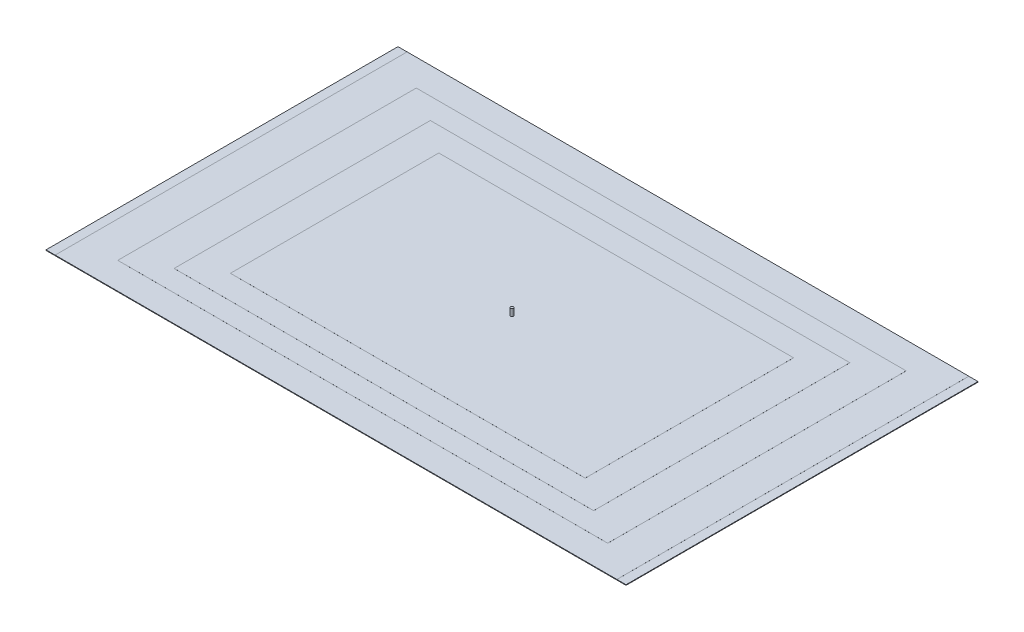
from build123d import *

# Parameters (mm, degrees)
SKETCH_1_W      = 2060
SKETCH_1_H      = 1250
EXTRUDE_1_DEPTH = 1
SKETCH_2_W      = 1995
SKETCH_2_H      = 1250
EXTRUDE_2_DEPTH = 0.1
SKETCH_3_W      = 1740
SKETCH_3_H      = 1060
EXTRUDE_5_DEPTH = 0.1
SKETCH_4_W      = 1490
SKETCH_4_H      = 910
EXTRUDE_6_DEPTH = 0.1
SKETCH_5_W      = 1260
SKETCH_5_H      = 740
EXTRUDE_7_DEPTH = 0.1
SKETCH_6_R      = 5
EXTRUDE_8_DEPTH = 25


with BuildPart() as part:
    # 草图1 → 凸台-拉伸1 (new, symmetric)
    with BuildSketch(Plane(origin=(0, 0, 0), x_dir=(1, 0, 0), z_dir=(0, 1, 0))):
        Rectangle(SKETCH_1_W, SKETCH_1_H)
    extrude(amount=EXTRUDE_1_DEPTH, both=True)


with BuildPart() as body_2:
    # 草图2 → 凸台-拉伸2 (new body)
    with BuildSketch(Plane(origin=(0, 1, 0), x_dir=(1, 0, 0), z_dir=(0, 1, 0))):
        Rectangle(SKETCH_2_W, SKETCH_2_H)
    extrude(amount=EXTRUDE_2_DEPTH)


with BuildPart() as body_3:
    # 草图3 → 凸台-拉伸5 (new body)
    with BuildSketch(Plane(origin=(0, 1.1, 0), x_dir=(1, 0, 0), z_dir=(0, 1, 0))):
        Rectangle(SKETCH_3_W, SKETCH_3_H)
    extrude(amount=EXTRUDE_5_DEPTH)


with BuildPart() as body_4:
    # 草图4 → 凸台-拉伸6 (new body)
    with BuildSketch(Plane(origin=(0, 1.2, 0), x_dir=(1, 0, 0), z_dir=(0, 1, 0))):
        Rectangle(SKETCH_4_W, SKETCH_4_H)
    extrude(amount=EXTRUDE_6_DEPTH)


with BuildPart() as body_5:
    # 草图5 → 凸台-拉伸7 (new body)
    with BuildSketch(Plane(origin=(0, 1.3, 0), x_dir=(1, 0, 0), z_dir=(0, 1, 0))):
        Rectangle(SKETCH_5_W, SKETCH_5_H)
    extrude(amount=EXTRUDE_7_DEPTH)

    # 草图6 → 凸台-拉伸8 (add, symmetric)
    with BuildSketch(Plane(origin=(0, 1.4, 0), x_dir=(1, 0, 0), z_dir=(0, 1, 0))):
        with Locations(Location((0, 0, 0), (0, 0, 90))):
            Circle(SKETCH_6_R)
    extrude(amount=EXTRUDE_8_DEPTH, both=True)


solid = Compound([part.part, body_2.part, body_3.part, body_4.part, body_5.part])
